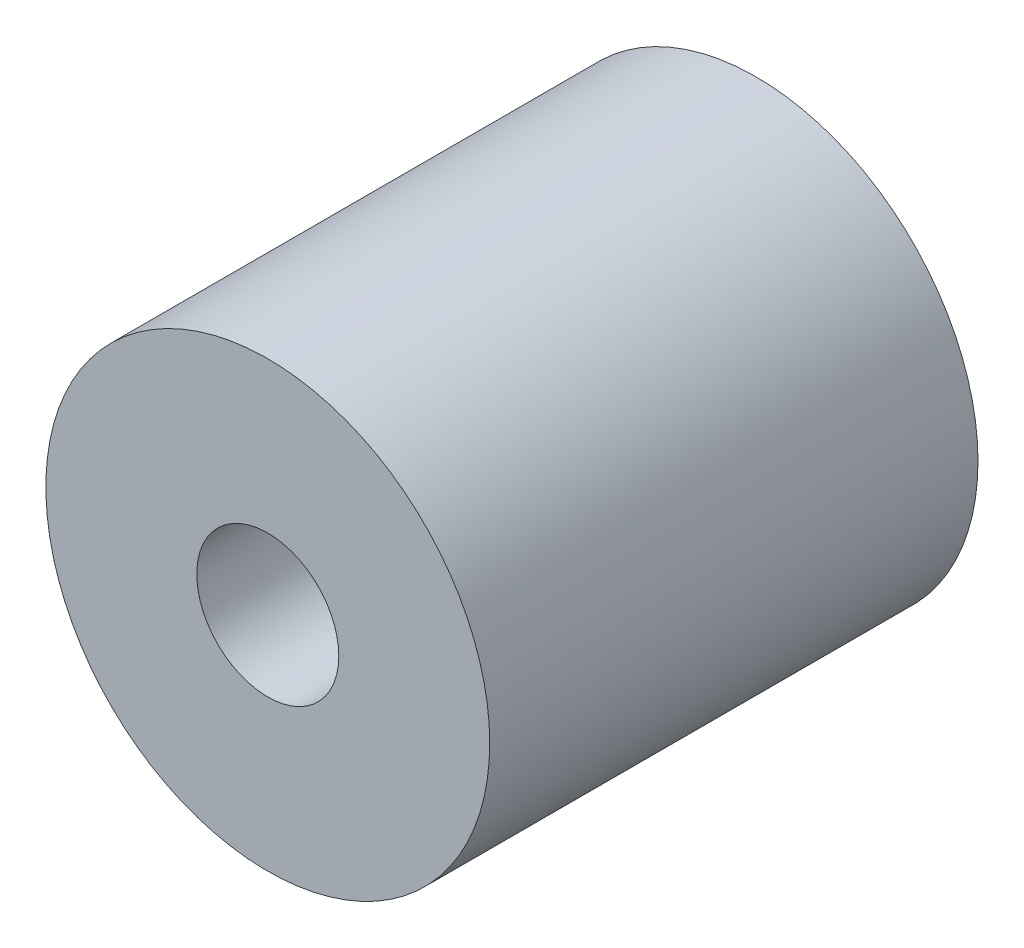
from build123d import *

# Parameters (mm, degrees)
SKETCH_1_R      = 10
SKETCH_1_R_2    = 3.2
EXTRUDE_1_DEPTH = 11


with BuildPart() as part:
    # 草图1 → 凸台-拉伸1 (new, symmetric)
    with BuildSketch(Plane.XY):
        Circle(SKETCH_1_R)
        Circle(SKETCH_1_R_2, mode=Mode.SUBTRACT)
    extrude(amount=EXTRUDE_1_DEPTH, both=True)


solid = part.part
